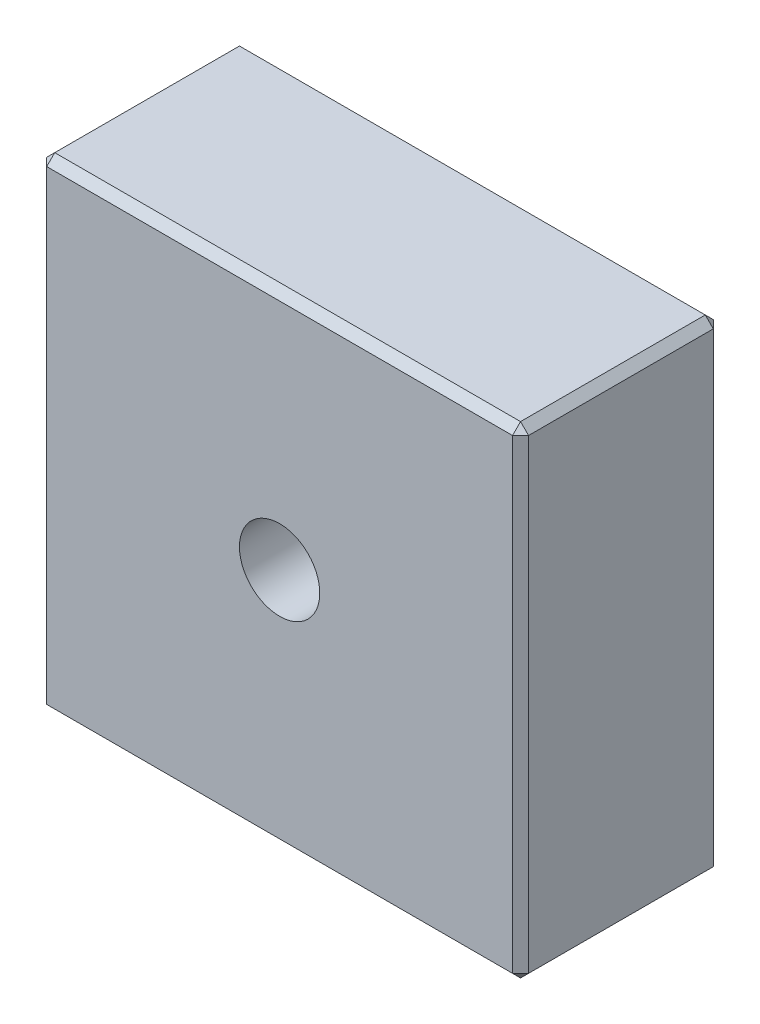
from build123d import *

# Parameters (mm, degrees)
SKETCH1_W           = 60
SKETCH1_H           = 60
BOSS_EXTRUDE1_DEPTH = 25
CHAMFER1_SIZE       = 1
SKETCH2_R           = 15
CUT_EXTRUDE1_DEPTH  = 7
SKETCH3_R           = 5
CUT_EXTRUDE2_DEPTH  = 47.086874487


with BuildPart() as part:
    # Sketch1 → Boss-Extrude1 (new body)
    with BuildSketch(Plane.XY):
        Rectangle(SKETCH1_W, SKETCH1_H)
    extrude(amount=BOSS_EXTRUDE1_DEPTH)

    # Chamfer1
    chamfer1_edges = [part.edges().sort_by_distance(p)[0] for p in [
        (30, 0, 25),
        (0, -30, 25),
        (-30, 0, 25),
        (0, -30, 0),
        (30, 0, 0),
        (0, 30, 0),
        (-30, 0, 0),
        (0, 30, 25),
        (-30, -30, 12.5),
        (30, -30, 12.5),
        (30, 30, 12.5),
        (-30, 30, 12.5),
    ]]
    chamfer(chamfer1_edges, length=CHAMFER1_SIZE)

    # Sketch2 → Cut-Extrude1 (cut)
    with BuildSketch(Plane(origin=(0, 0, 0), x_dir=(-1, 0, 0), z_dir=(0, 0, -1))):
        Circle(SKETCH2_R)
    extrude(amount=-CUT_EXTRUDE1_DEPTH, mode=Mode.SUBTRACT)

    # Sketch3 → Cut-Extrude2 (cut, through all)
    with BuildSketch(Plane(origin=(0, 0, 7), x_dir=(-1, 0, 0), z_dir=(0, 0, -1))):
        Circle(SKETCH3_R)
    extrude(amount=-CUT_EXTRUDE2_DEPTH, mode=Mode.SUBTRACT)


solid = part.part
